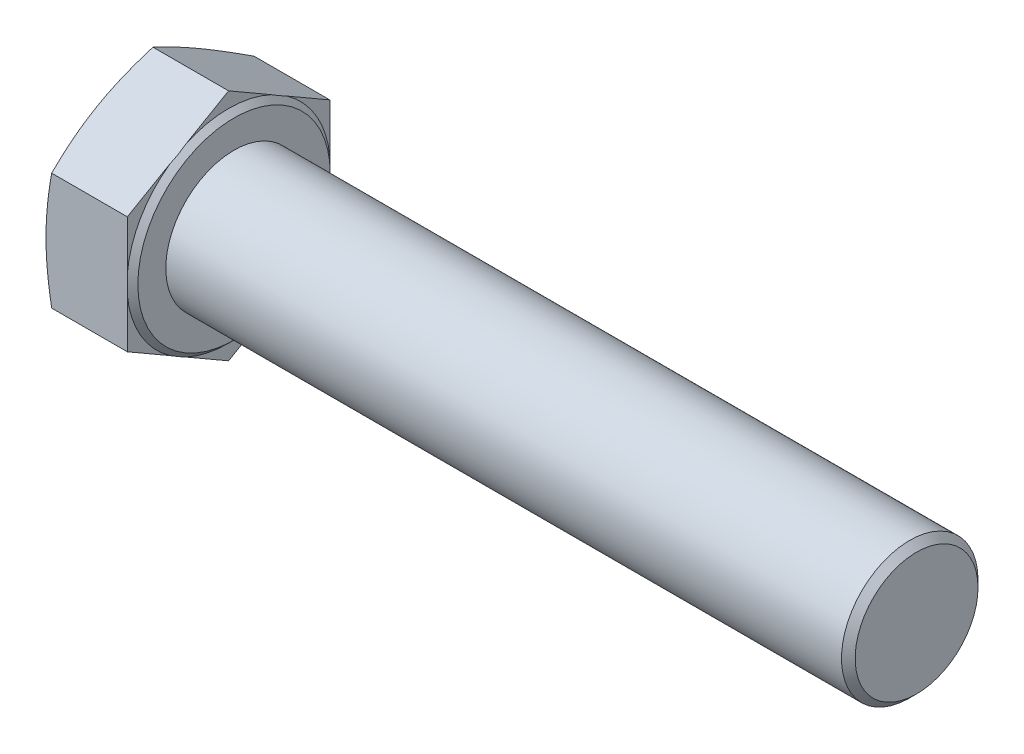
from build123d import *

# Parameters (mm, degrees)
BASEHEAD_DEPTH = 12.715
SKETCH5_R      = 10
BASEBODY_DEPTH = 100
CHAMFER1_SIZE  = 1


with BuildPart() as part:
    # Sketch2 → BaseHead (new body)
    with BuildSketch(Plane(origin=(0, 0, 0), x_dir=(0, 0, -1), z_dir=(1, 0, 0))):
        Polygon((14.835, -8.564991243), (14.835, 8.564991243), (0, 17.129982487), (-14.835, 8.564991243), (-14.835, -8.564991243), (0, -17.129982487), align=None)
    extrude(amount=BASEHEAD_DEPTH)

    # Sketch3 → BearingFace (revolve, cut)
    with BuildSketch(Plane.XY, mode=Mode.PRIVATE) as bearingface_sk:
        Polygon((12.715, 17.129982487), (12.715, 14.095), (11.915, 14.895), (11.915, 17.129982487), align=None)
    revolve(bearingface_sk.sketch.rotate(Axis((-0.957090588, 0, 0), (1, 0, 0)), 90), axis=Axis((-0.957090588, 0, 0), (1, 0, 0)), mode=Mode.SUBTRACT)

    # Sketch4 → HeadChamfer (revolve, cut)
    with BuildSketch(Plane.XY):
        Polygon((0, 17.129982487), (0.835305313, 17.129982487), (0, 14.835), align=None)
    revolve(axis=Axis((-0.493528746, 0, 0), (1, 0, 0)), mode=Mode.SUBTRACT)

    # Sketch5 → BaseBody (add)
    with BuildSketch(Plane(origin=(12.715, 0, 0), x_dir=(0, 0, -1), z_dir=(1, 0, 0))):
        Circle(SKETCH5_R)
    extrude(amount=BASEBODY_DEPTH)

    # Chamfer1
    chamfer1_edges = [part.edges().sort_by_distance(p)[0] for p in [
        (112.715, 0, 10),
    ]]
    chamfer(chamfer1_edges, length=CHAMFER1_SIZE)


solid = part.part
